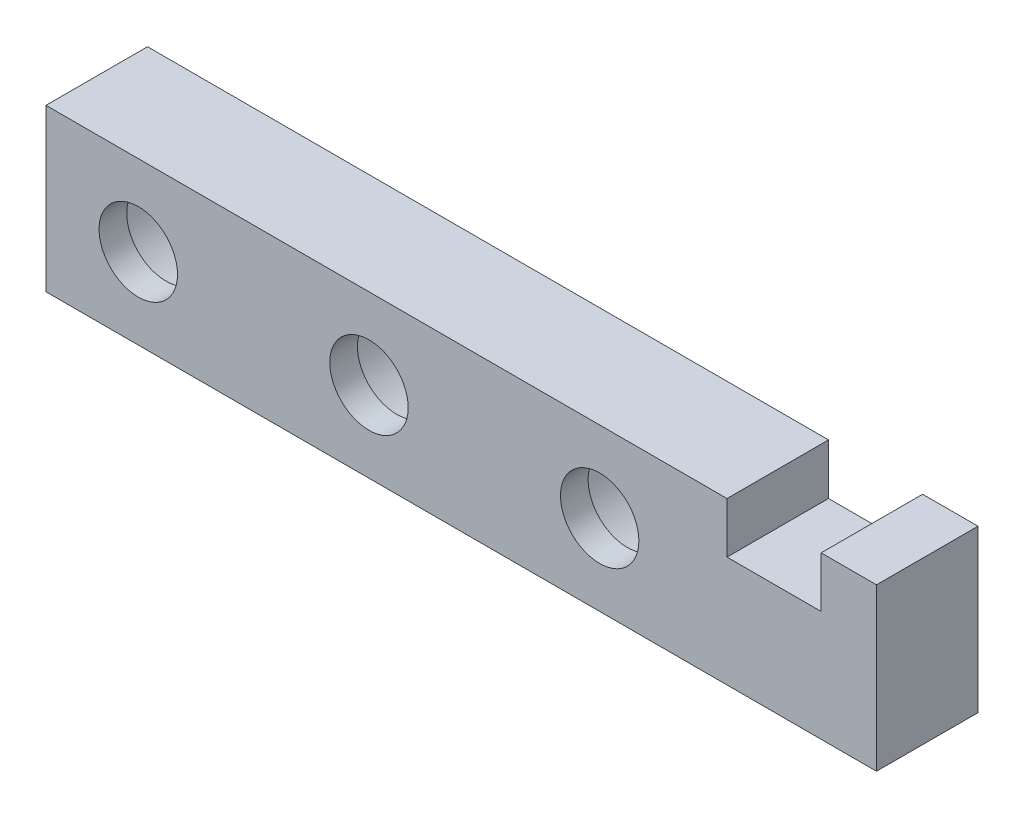
SolidWorks part; units mm, degrees
ref_plane "Front Plane" through (0, 0, 0) normal (0, 0, 1) x (1, 0, 0)
ref_plane "Top Plane" through (0, 0, 0) normal (0, 1, 0) x (1, 0, 0)
ref_plane "Right Plane" through (0, 0, 0) normal (1, 0, 0) x (0, 0, -1)
sketch "Sketch1" plane through (0, 0, 0) normal (0, 0, 1) x (1, 0, 0)
  line L0 (-45, 0) -> (45, 0) construction
  line L1 (-45, 8.75) -> (28.8, 8.75)
  line L2 (-45, 8.75) -> (-45, -8.75)
  line L3 (-45, -8.75) -> (45, -8.75)
  line L4 (45, 8.75) -> (45, -8.75)
  line L5 (-45, 8.75) -> (45, -8.75) construction
  line L6 (-45, -8.75) -> (45, 8.75) construction
  line L7 (28.8, 8.75) -> (28.8, 3.25)
  line L8 (28.8, 3.25) -> (39, 3.25)
  line L9 (39, 3.25) -> (39, 8.75)
  line L10 (39, 8.75) -> (45, 8.75)
  circle A0 centre (-35, 0) radius 4.25
  circle A1 centre (-10, 0) radius 4.25
  circle A2 centre (15, 0) radius 4.25
  point P0 (0, 0)
  dimension "D3" = 8.5
  dimension "D4" = 8.5
  dimension "D5" = 8.5
  dimension "D6" = 30
  dimension "D7" = 25
  dimension "D8" = 25
  dimension "D1" = 90
  dimension "D2" = 17.5
  dimension "D9" = 6
  dimension "D10" = 10.2
  dimension "D11" = 5.5
extrude "Boss-Extrude1" add sketch "Sketch1" along normal blind 11
sketch "Sketch2" plane through (0, 0, 11) normal (0, 0, 1) x (1, 0, 0)
  circle A0 centre (-35, 0) radius 7.5
  circle A1 centre (-10, 0) radius 7.5
  circle A2 centre (15, 0) radius 7.5
  dimension "D1" = 15
  dimension "D2" = 15
  dimension "D3" = 15
extrude "Cut-Extrude1" cut sketch "Sketch2" against normal blind 8 from offset 3
